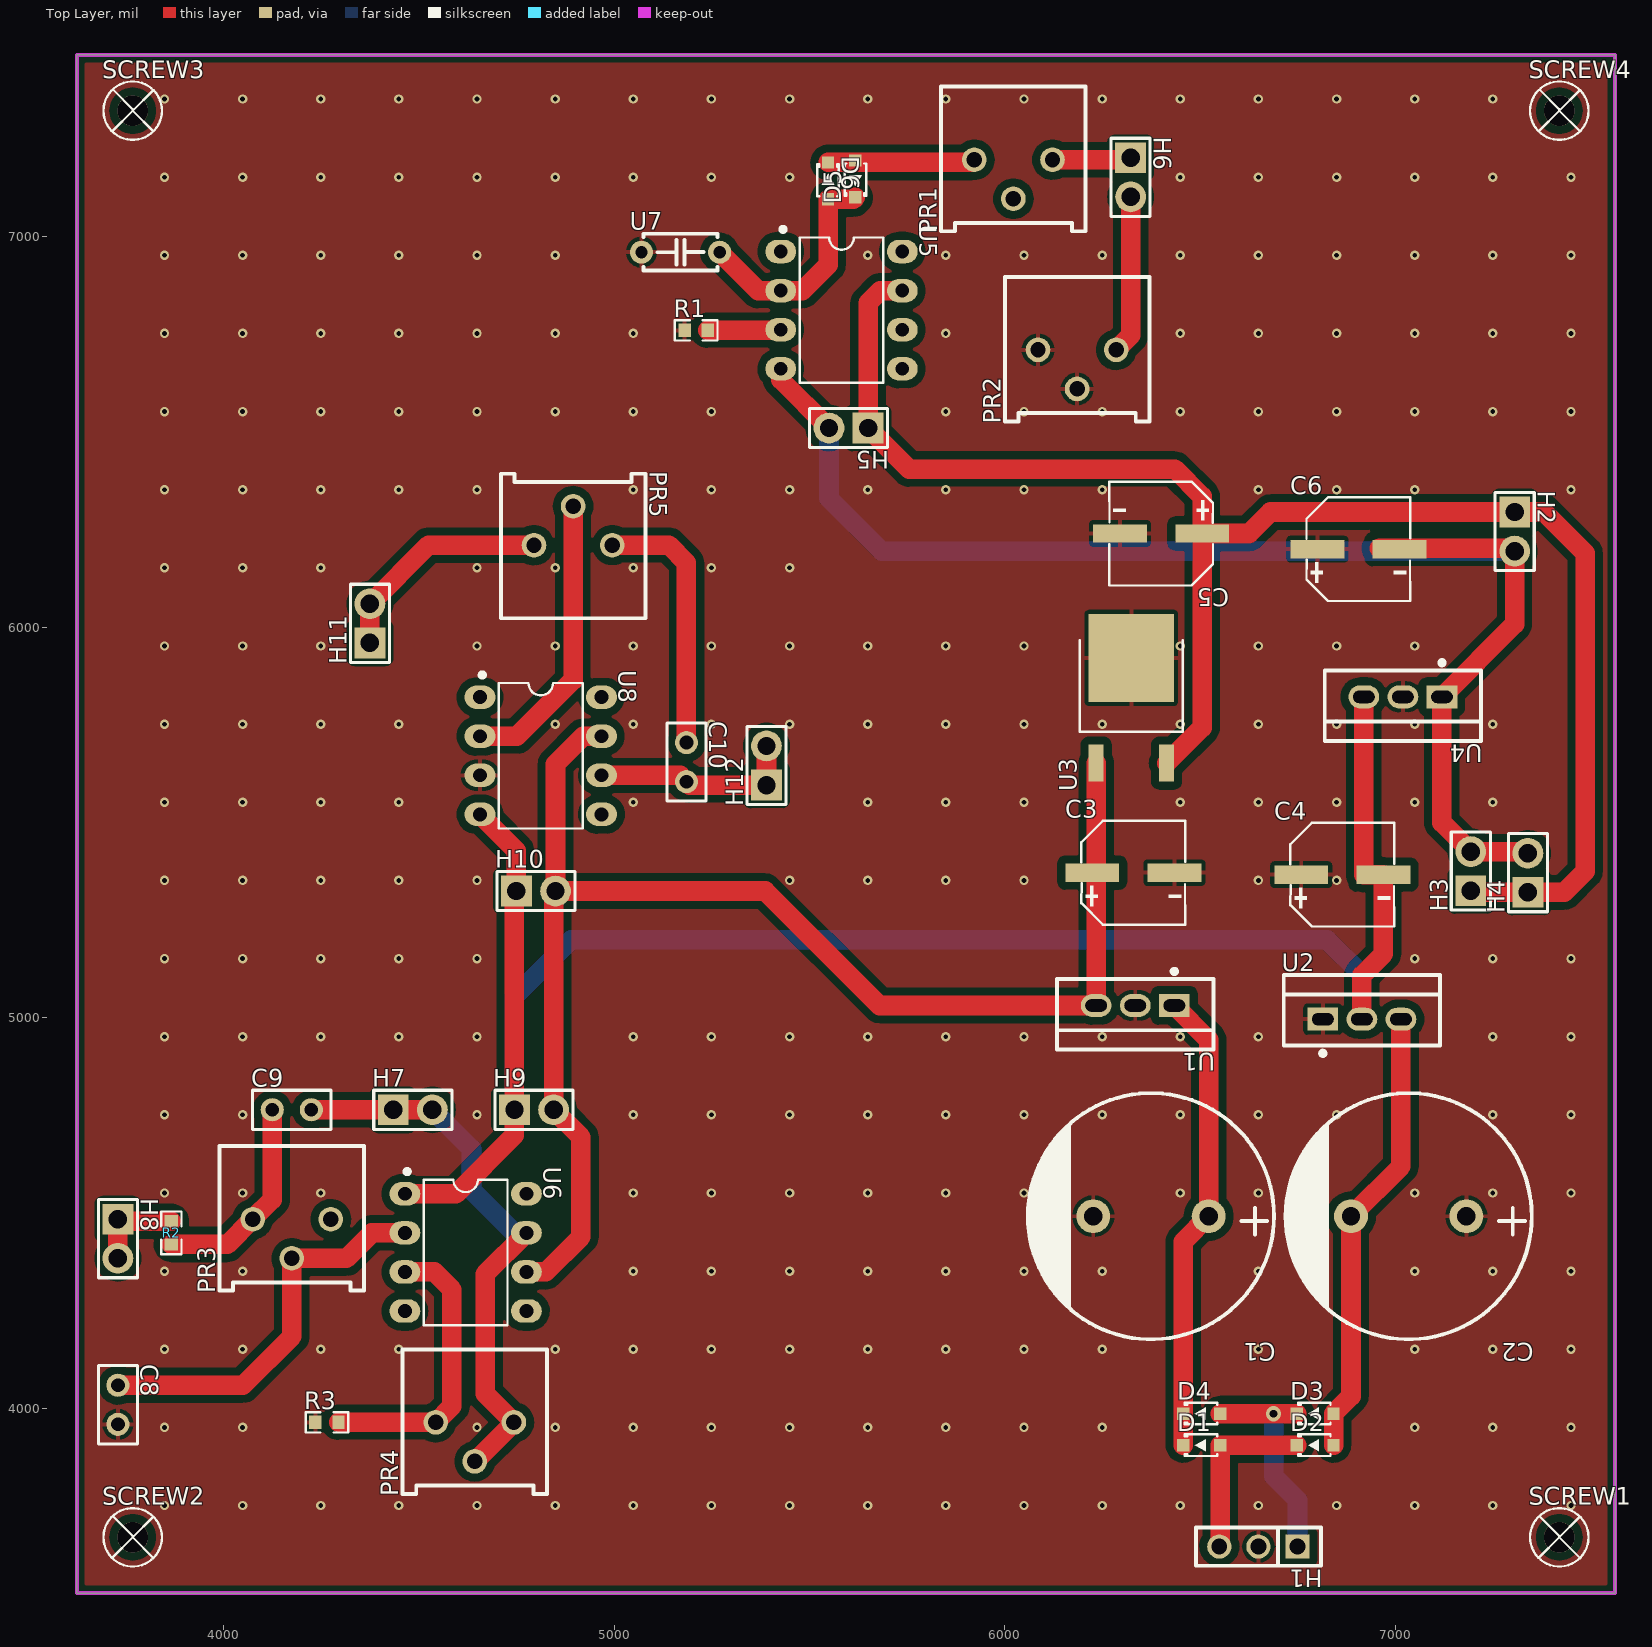
[diagram p0: Top Layer view]
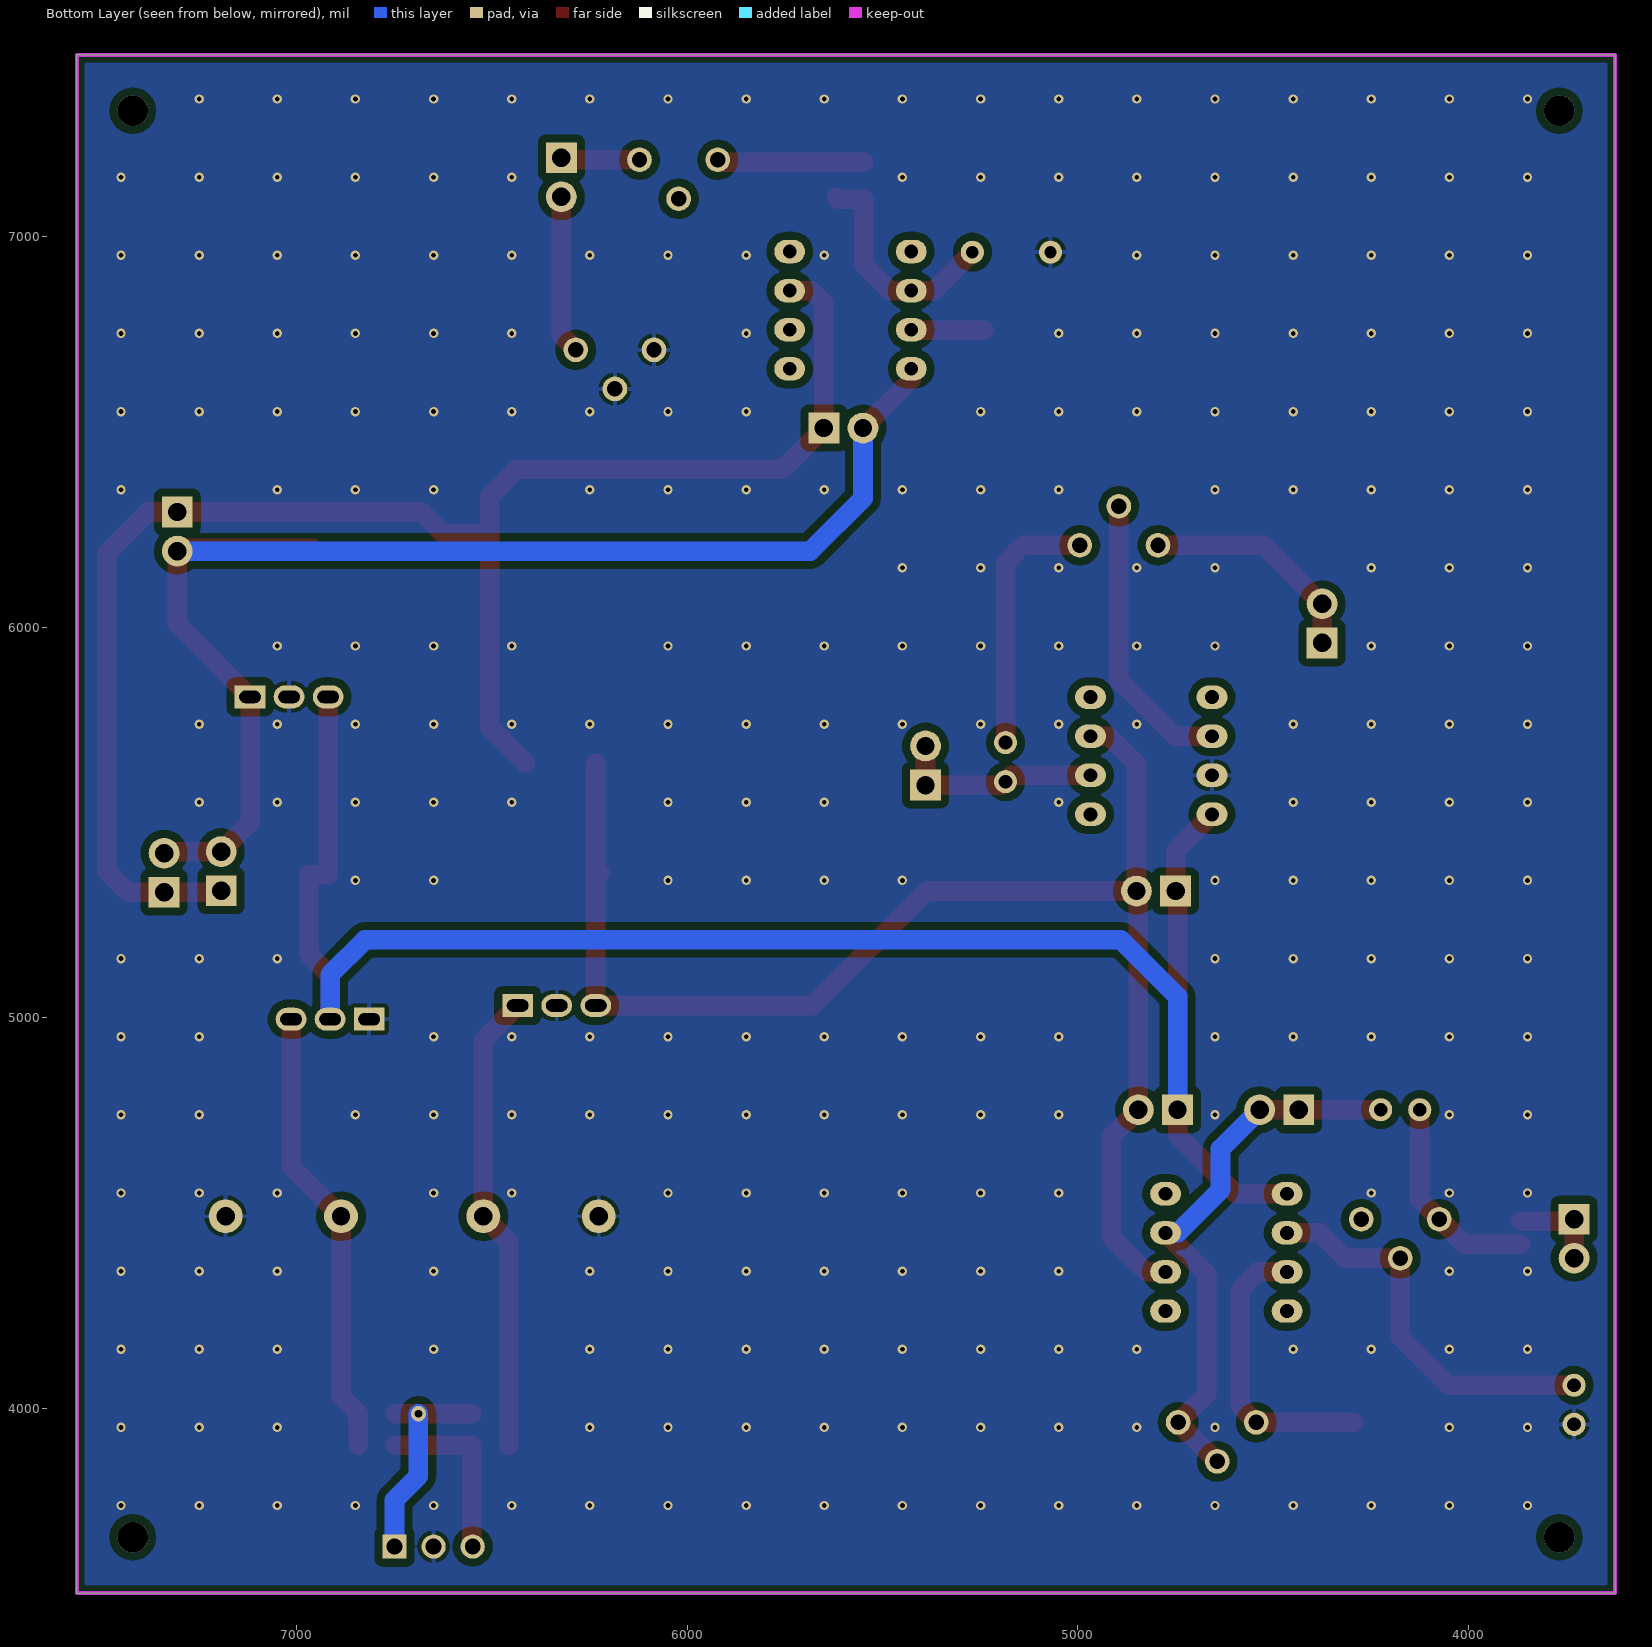
[diagram p1: Bottom Layer view, seen from below]
# Altium PCB MISC75076.pcbdoc
Units mil, origin at the board's own origin, x right, y up, seen from the top; angles counter-clockwise.
Board outline 3937.01 x 3937.01 mil, 2 copper layers (Top Layer, Bottom Layer), stack 62.206 mil thick; 47 components, 23 nets, 118 pads, 276 vias.

## Layer stack, top to bottom
Top Solder Mask Layer: solder mask 0.394, Dk 3.3
Top Layer: signal copper 1.379
Dielectric1: surface 59.449, FR4, Dk 4.5
Bottom Layer: signal copper 1.378
Bottom Solder Mask Layer: solder mask 0.394, Dk 3.3

## Board outline
3625,7465 3625,3527.99 7562.01,3527.99 7562.01,7465

## Design rules (kind name [scope] priority, off if disabled: settings)
BoardOutlineClearance copperThickness2oz_1 [All] p2 off: genericclearance=8 ignorepadtopadclearanceinfootprint=FALSE except(0: Arc-SplitContinuation Track-SplitContinuation SMDPad-SplitContinuation THPad-SplitContinuation Via-SplitContinuation Fill-SplitContinuation Region-SplitContinuation Poly-SplitContinuation Text-SplitContinuation Hole-SplitContinuation; 6: Arc-CutoutEdge Track-CutoutEdge SMDPad-CutoutEdge THPad-CutoutEdge Via-CutoutEdge Text-CutoutEdge; 6.9: Hole-OutlineEdge Hole-CutoutEdge; 11.8: Arc-OutlineEdge Track-OutlineEdge SMDPad-OutlineEdge THPad-OutlineEdge Via-OutlineEdge Fill-OutlineEdge Region-OutlineEdge Text-OutlineEdge Fill-CutoutEdge Region-CutoutEdge; 20: Poly-OutlineEdge Poly-CutoutEdge)
BoardOutlineClearance Copper_copperRegion_1 [All] p4 off: genericclearance=8 ignorepadtopadclearanceinfootprint=FALSE except(0: Arc-SplitContinuation Track-SplitContinuation SMDPad-SplitContinuation THPad-SplitContinuation Via-SplitContinuation Fill-SplitContinuation Region-SplitContinuation Poly-SplitContinuation Text-SplitContinuation Hole-SplitContinuation; 8: Arc-OutlineEdge Track-OutlineEdge SMDPad-OutlineEdge THPad-OutlineEdge Via-OutlineEdge Fill-OutlineEdge Region-OutlineEdge Text-OutlineEdge Hole-OutlineEdge Arc-CutoutEdge Track-CutoutEdge SMDPad-CutoutEdge THPad-CutoutEdge Via-CutoutEdge Fill-CutoutEdge Region-CutoutEdge Text-CutoutEdge Hole-CutoutEdge; 20: Poly-OutlineEdge Poly-CutoutEdge)
BoardOutlineClearance Plane_innerPlane_1 [All] p6 off: genericclearance=8 ignorepadtopadclearanceinfootprint=FALSE except(0: Arc-SplitContinuation Track-SplitContinuation SMDPad-SplitContinuation THPad-SplitContinuation Via-SplitContinuation Fill-SplitContinuation Region-SplitContinuation Poly-SplitContinuation Text-SplitContinuation Hole-SplitContinuation; 8: Arc-OutlineEdge Track-OutlineEdge SMDPad-OutlineEdge THPad-OutlineEdge Via-OutlineEdge Fill-OutlineEdge Region-OutlineEdge Text-OutlineEdge Hole-OutlineEdge Arc-CutoutEdge Track-CutoutEdge SMDPad-CutoutEdge THPad-CutoutEdge Via-CutoutEdge Fill-CutoutEdge Region-CutoutEdge Text-CutoutEdge Hole-CutoutEdge; 10: Poly-OutlineEdge Poly-CutoutEdge)
BoardOutlineClearance copperThickness1oz_1 [All] p8: genericclearance=8 ignorepadtopadclearanceinfootprint=FALSE except(0: Arc-SplitContinuation Track-SplitContinuation SMDPad-SplitContinuation THPad-SplitContinuation Via-SplitContinuation Fill-SplitContinuation Region-SplitContinuation Poly-SplitContinuation Text-SplitContinuation Hole-SplitContinuation; 8: Arc-OutlineEdge Track-OutlineEdge SMDPad-OutlineEdge THPad-OutlineEdge Via-OutlineEdge Fill-OutlineEdge Region-OutlineEdge Text-OutlineEdge Hole-OutlineEdge Arc-CutoutEdge Track-CutoutEdge SMDPad-CutoutEdge THPad-CutoutEdge Via-CutoutEdge Fill-CutoutEdge Region-CutoutEdge Text-CutoutEdge Hole-CutoutEdge; 20: Poly-OutlineEdge Poly-CutoutEdge)
Clearance copperThickness2oz [All] p1 off: gap=8 ignorepadtopadclearanceinfootprint=FALSE except(6: SMDPad-Track SMDPad-SMDPad THPad-Track SMDPad-THPad THPad-THPad Track-Via SMDPad-Via THPad-Via Via-Via Fill-SMDPad Region-SMDPad Fill-THPad Region-THPad Fill-Via Region-Via Fill-Fill Fill-Region Region-Region Arc-Track Arc-SMDPad Arc-THPad Arc-Via Fill-Arc Region-Arc Arc-Arc Text-Track SMDPad-Text Text-THPad Text-Via Fill-Text Region-Text Arc-Text Text-Text; 6.9: Hole-Track Hole-SMDPad Hole-THPad Hole-Via Fill-Hole Region-Hole Hole-Arc Hole-Text; 11.8: Fill-Track Region-Track; 20: Poly-Track Poly-SMDPad Poly-THPad Poly-Via Poly-Fill Poly-Region Poly-Poly Poly-Arc Poly-Text Poly-Hole)
Clearance Copper_copperRegion [All] p3 off: gap=8 ignorepadtopadclearanceinfootprint=FALSE except(20: Poly-Track Poly-SMDPad Poly-THPad Poly-Via Poly-Fill Poly-Region Poly-Poly Poly-Arc Poly-Text Poly-Hole)
Clearance Plane_innerPlane [All] p5 off: gap=8 ignorepadtopadclearanceinfootprint=FALSE except(10: Poly-Track Poly-SMDPad Poly-THPad Poly-Via Poly-Fill Poly-Region Poly-Poly Poly-Arc Poly-Text Poly-Hole)
Clearance copperThickness1oz [All] p7: gap=8 ignorepadtopadclearanceinfootprint=FALSE except(20: Poly-Track Poly-SMDPad Poly-THPad Poly-Via Poly-Fill Poly-Region Poly-Poly Poly-Arc Poly-Text Poly-Hole)
DiffPairsRouting differentialPair [All] p1: maxlimit=6 minlimit=6 mostfreqgap=6 toplayer_minwidth=5 toplayer_prefwidth=10 toplayer_maxwidth=100 toplayer_mingap=6 toplayer_prefgap=6 toplayer_maxgap=6 bottomlayer_minwidth=5 bottomlayer_prefwidth=10 bottomlayer_maxwidth=100 bottomlayer_mingap=6 bottomlayer_prefgap=6 bottomlayer_maxgap=6 maxuncoupledlength=10
HoleToHoleClearance otherClearance [All] p1: gap=11.8 allowstackedmicrovias=TRUE
Length netLength [All] p1: minlimit=0 maxlimit=0
MatchedLengths netLengthTolerance [All] p1: tolerance=1000
PasteMaskExpansion pasteMaskExpansion [All] p1: expansion=0
PlaneConnect innerPlane [All] p1: planeconnectstyle=Relief reliefexpansion=20 reliefentries=4 reliefconductorwidth=10 reliefairgap=10
PolygonConnect copperRegion [(InNet('GND'))] p1: connectstyle=Relief reliefconductorwidth=10 reliefentries=4 polygonreliefangle="90 Angle" airgapwidth=10 via.connectstyle=Relief via.reliefconductorwidth=10 via.reliefentries=4 via.polygonreliefangle="90 Angle" via.airgapwidth=10
RoutingVias viaSize [All] p1: holewidth=12 width=24 viastyle="Through Hole" minholewidth=11.8 minwidth=19.7 maxholewidth=248 maxwidth=393.7
SolderMaskExpansion solderMaskExpansion [IsVia] p1: expansion=-1000 istentingtop=TRUE
SolderMaskExpansion solderMaskExpansion [All] p2: expansion=2 istentingtop=FALSE
Width copperThickness2oz_2 [(InNet('-5V') OR InNet('-12V') OR InNet('+5V') OR InNet('+12V'))] p1: maxlimit=100 minlimit=8 preferedwidth=10
Width "VCC and GND" [All] p2 off: maxlimit=30 minlimit=10 preferedwidth=30
Width copperThickness1oz_2 [All] p3: maxlimit=50 minlimit=8 preferedwidth=50

## Components (designator, comment, footprint, x,y, rotation, side; value= is the part's Value field where it differs from the comment)
C1 "2200uF" CAP-TH_BD16.0-P7.50-D0.8-FD 6374.05,4492.61 r180 top
C2 "2200uF" CAP-TH_BD16.0-P7.50-D0.8-FD 7033.66,4492.61 r180 top
C3 "330uF" CAP-SMD_BD6.3-L6.6-W6.6-LS7.2-FD_3 6328.86,5371.91 r0 top
C4 "330uF" CAP-SMD_BD6.3-L6.6-W6.6-LS7.2-FD_3 6863.86,5366.91 r0 top
C5 "100uF" CAP-SMD_BD6.3-L6.6-W6.6-LS7.3-FD-H7.7 6400,6240 r180 top
C6 "100uF" CAP-SMD_BD6.3-L6.6-W6.6-LS7.3-FD-H7.7 6905,6200 r0 top
C8 "100nF" CAP-TH_L5.0-W2.5-P2.54-D0.7 3730,4010 r270 top
C9 "100nF" CAP-TH_L5.0-W2.5-P2.54-D0.7 4175,4765.15 r0 top
C10 "100nF" CAP-TH_L5.0-W2.5-P2.54-D0.7 5185.2,5654.8 r270 top
D1 "1N4007WS" SOD-323_L1.7-W1.3-LS2.5-RD 6504.05,3906.62 r0 top
D2 "1N4007WS" SOD-323_L1.7-W1.3-LS2.5-RD 6794.05,3906.62 r0 top
D3 "1N4007WS" SOD-323_L1.7-W1.3-LS2.5-RD 6794.05,3987.4 r0 top
D4 "1N4007WS" SOD-323_L1.7-W1.3-LS2.5-RD 6504.05,3987.4 r0 top
D5 "1N4007WS" SOD-323_L1.7-W1.3-LS2.5-RD 5617.5,7147.5 r90 top
D6 "1N4007WS" SOD-323_L1.7-W1.3-LS2.5-RD 5547.5,7142.5 r270 top
H1 "PM254V-11-03-H85" HDR-TH_3P-P2.54-V-F 6649.05,3647.17 r180 top
H2 "HX PH254-01-02-Z-L11.5 male header connector" HDR-TH_2P-P2.54-V-M 7305,6245 r270 top
H3 "HX PH254-01-02-Z-L11.5 male header connector" HDR-TH_2P-P2.54-V-M 7192.74,5375.94 r90 top
H4 "HX PH254-01-02-Z-L11.5 male header connector" HDR-TH_2P-P2.54-V-M 7338.86,5371.91 r90 top
H5 "HX PH254-01-02-Z-L11.5 male header connector" HDR-TH_2P-P2.54-V-M 5600,6510 r180 top
H6 "HX PH254-01-02-Z-L11.5 male header connector" HDR-TH_2P-P2.54-V-M 6322,7151.59 r270 top
H7 "HX PH254-01-02-Z-L11.5 male header connector" HDR-TH_2P-P2.54-V-M 4484.93,4765 r0 top
H8 "HX PH254-01-02-Z-L11.5 male header connector" HDR-TH_2P-P2.54-V-M 3730,4435 r270 top
H9 "HX PH254-01-02-Z-L11.5 male header connector" HDR-TH_2P-P2.54-V-M 4795,4765 r0 top
H10 "HX PH254-01-02-Z-L11.5 male header connector" HDR-TH_2P-P2.54-V-M 4800,5325 r0 top
H11 "HX PH254-01-02-Z-L11.5 male header connector" HDR-TH_2P-P2.54-V-M 4375,6010 r90 top
H12 "HX PH254-01-02-Z-L11.5 male header connector" HDR-TH_2P-P2.54-V-M 5389.98,5646.15 r90 top
PR1 "5K" R_3386P 6022,7196.59 r90 top
PR2 "5K" R_3386P 6185,6710 r90 top
PR3 "1K" R_3386P 4175,4485 r90 top
PR4 "1K" R_3386P 4643.49,3965 r90 top
PR5 "2K" R_3386P 4895,6210 r270 top
R1 "1kΩ" R0603 5210,6760 r0 top
R2 "1kΩ" R0603 3866.78,4450 r270 top
R3 "1kΩ" R0603 4265,3965 r0 top
SCREW1 "" M2螺丝 7419.15,3670.85 r0 top
SCREW2 "" M2螺丝 3767.85,3670.85 r0 top
SCREW3 "" M2螺丝 3767.85,7322.15 r0 top
SCREW4 "" M2螺丝 7419.15,7322.15 r0 top
U1 "LM7812CT/NOPB" TO-220-3_L10.2-W4.6-P2.54-L 6333.86,5031.91 r180 top
U2 "LM7912CT/NOPB" TO-220-3_L10.2-W4.6-P2.54-L 6913.86,4996.91 r0 top
U3 "LM7805-5V" TO-252-2_L6.6-W6.1-P4.58-LS9.9-TL 6323.86,5786.91 r90 top
U4 "LM7812CT/NOPB" TO-220-3_L10.2-W4.6-P2.54-L 7018.86,5821.91 r180 top
U5 "LF411CP" PDIP-8_L9.3-W6.4-P2.54-LS7.9-BL-1 5582,6811.59 r270 top
U6 "LF411CP" PDIP-8_L9.3-W6.4-P2.54-LS7.9-BL-1 4620,4400 r270 top
U7 "470nF" CAP-TH_L4.8-W2.4-P5.08-D0.6 5170,6960 r0 top
U8 "LF411CP" PDIP-8_L9.3-W6.4-P2.54-LS7.9-BL-1 4812.25,5671.15 r270 top

## Footprints (in the part's own frame and the unit in brackets; to place one, negate y for a bottom-side part, rotate by r counter-clockwise, add the part's x,y. Pads: shape width x height; smd on the part's side, far side on the other; paste and mask are expansions set on the pad)
CAP-SMD_BD6.3-L6.6-W6.6-LS7.2-FD_3 [mm]
  rect 3.5x1.2 smd: 1(-2.67,0) 2(2.67,0)
  silkscreen extent -3.38,-3.38 3.38,3.38
CAP-SMD_BD6.3-L6.6-W6.6-LS7.3-FD-H7.7 [mm]
  rect 3.5x1.2 smd: 1(-2.67,0) 2(2.67,0)
  silkscreen extent -3.38,-3.38 3.38,3.38
CAP-TH_BD16.0-P7.50-D0.8-FD [mm]
  round 2.2 hole 1.2: 1(-3.75,0) 2(3.75,0)
  silkscreen extent -8,-8 8,8
CAP-TH_L4.8-W2.4-P5.08-D0.6 [mm]
  round 1.5 hole 0.8: 1(-2.54,0) 2(2.54,0)
  silkscreen extent -2.4,-1.2 2.4,1.2
CAP-TH_L5.0-W2.5-P2.54-D0.7 [mm]
  round 1.5 hole 0.9 paste+0 mask+0.05: 1(-1.27,0) 2(1.27,0)
  silkscreen extent -2.54,-1.27 2.54,1.27
HDR-TH_2P-P2.54-V-M [mm]
  rect 2x2 hole 1.2: 1(-1.27,0)
  round 2 hole 1.2: 2(1.27,0)
  silkscreen extent -2.54,-1.27 2.54,1.27
HDR-TH_3P-P2.54-V-F [mil]
  rect 62x62 hole 40.16: 1(-100,0)
  round 62 hole 40.16: 2(0,0) 3(100,0)
  silkscreen extent -160,-49 160,49
M2螺丝 [mm]
  round 2 hole 2: 1(0,0)
  silkscreen extent -1.9,-1.9 1.9,1.9
PDIP-8_L9.3-W6.4-P2.54-LS7.9-BL-1 [mm]
  oval 1.524x2 hole 0.9: 1(-3.81,-3.95) 2(-1.27,-3.95) 3(1.27,-3.95) 4(3.81,-3.95) 5(3.81,3.95) 6(1.27,3.95) 7(-1.27,3.95) 8(-3.81,3.95)
  silkscreen extent -5.4,-3.95 4.73,2.72
R0603 [mil]
  rect 31.75x34.02 smd paste-3937.01 mask+2: 1(-29.66,0) 2(29.66,0)
  silkscreen extent -55,-26 55,26
R_3386P [mil]
  round 63 hole 39.4 paste+0 mask+2: 1(0,-100) 2(-100,0) 3(0,100)
  silkscreen extent -183,-185 187,185
SOD-323_L1.7-W1.3-LS2.5-RD [mm]
  rect 0.8x0.8 smd: 1(-1.2,0) 2(1.2,0)
  silkscreen extent -1.1,-0.7 1,0.7
TO-220-3_L10.2-W4.6-P2.54-L [mm]
  rect 2x1.5 hole 0.8 slot 1.4 at 0 deg: 1(-2.54,0)
  oval 2x1.5 hole 0.8 slot 1.4 at 0 deg: 2(0,0) 3(2.54,0)
  silkscreen extent -5.08,-2.37 5.08,2.86
TO-252-2_L6.6-W6.1-P4.58-LS9.9-TL [mil]
  rect 94.84x38.53 smd: 1(-134.8,90.15) 3(-134.78,-90.16)
  rect 224.84x218.44 smd: 2(134.8,0.01)
  silkscreen extent -54,-132 180,132

## Via types
v1: diameter 24, hole 12, Top Layer to Bottom Layer, 275 vias
v2: diameter 39.37, hole 19.7, Top Layer to Bottom Layer, 1 vias

## Nets (pads, with @x,y where several pads share a name; then routed paths per layer and width w, separated by ;. In a path a pad name is that pad's centre, name@x,y a point inside that pad or via, vN(x,y) a via of type N, cw(c..) or ccw(c..) an arc to the next point about the centre after c; other vN are vias at no path point)
$1N34: D1.2 D2.1 H1.3 | length 455.9
  Top Layer w50: H1.3 6551.29,3649.41 D1.2 D2.1
$1N35: D3.1 D4.2 H1.1 | length 561.2
  Top Layer w50: D4.2 v2(6687.74,3987.4) D3.1
  Bottom Layer w50: v2(6687.74,3987.4) 6687.74,3827.26 6749.05,3765.95 H1.1
$1N37: C1.1 D1.1 D4.1 U1.1 | length 1188.5
  Top Layer w50: U1.1 6521.69,4944.07 C1.1 6456.81,4427.73 D4.1 D1.1
$1N38: C2.2 D2.2 D3.2 U2.3 | length 1161.8
  Top Layer w50: D2.2 D3.2 6886.02,4032.13 C2.2 7013.86,4620.44 U2.3
$1N53: D5.1 D6.2 U5.2 U7.2 | length 585.4
  Top Layer w50: U7.2 5368.41,6861.59 U5.2 5481.59,6861.59 5547.5,6927.5 D6.2 5612.5,7095.26 D5.1
$1N54: R1.2 U5.3 | length 187.5
  Top Layer w50: R1.2 5424.9,6760 U5.3
$1N60: H6.2 PR2.1 | length 406.9
  Top Layer w50: PR2.1 6322,6747 H6.2
$1N61: D5.2 D6.1 PR1.3 | length 377.3
  Top Layer w50: D6.1 5915.15,7189.74 PR1.3
$1N67: H8.1 H8.2 R2.1 | length 239
  Top Layer w50: H8.2 H8.1 3735.34,4479.66 R2.1
$1N68: C9.1 PR3.3 R2.2 | length 535.9
  Top Layer w50: R2.2 4010.34,4420.34 PR3.3 4125,4535 C9.1
$1N70: PR4.3 R3.2 U6.3 | length 745.2
  Top Layer w50: R3.2 PR4.3 4585,4006.51 4585,4305 4540,4350 U6.3
$1N71: C8.1 PR3.2 U6.2 | length 1013.2
  Top Layer w50: C8.1 4050,4060 4175,4185 PR3.2 4315,4385 4380,4450 U6.2
$1N79: PR5.2 U8.2 | length 742.8
  Top Layer w50: U8.2 4751.15,5721.15 4895,5865 PR5.2
$1N80: H11.1 H11.2 PR5.1 | length 582.1
  Top Layer w50: H11.1 H11.2 4525,6210 PR5.1
$1N81: C10.1 PR5.3 | length 668.9
  Top Layer w50: PR5.3 5140,6210 5185.2,6164.8 C10.1
+5V: C5.1 H2.1 H3.1 H4.1 H5.1 U3.3 U5.7 | length 4245.8
  Top Layer w50: U5.7 5681.59,6861.59 5650,6830 H5.1 5755,6405 6435,6405 6505.12,6334.88 C5.1 ; U3.3 6505.12,5743.24 C5.1 ; H3.1 7196.77,5321.91 H4.1 7431.91,5321.91 7485,5375 7485,6190 7380,6295 H2.1 6680,6295 6625,6240 C5.1
+12V: C3.1 H9.2 H10.2 U1.3 U3.1 U6.6 U8.7 | length 3704.7
  Top Layer w50: U6.6 4825,4350 4915,4440 4915,4695 H9.2 4845,5320 H10.2 ; U8.7 4921.15,5721.15 4850,5650 H10.2 ; C3.1 C3.1@6233.7,5381.87 ; U3.1 C3.1@6233.7,5381.87 ; H10.2 5386.25,5325 5679.34,5031.92 U1.3 6233.7,5032.07 C3.1@6233.7,5381.87
-5V: C6.2 H2.2 H3.2 H4.2 H5.2 U4.1 U5.4 | length 3567.1
  Top Layer w50: U5.4 5426.49,6633.51 H5.2 ; C6.2@6958.98,6201.91 7298.09,6201.91 H2.2 7305,6008.05 U4.1 7118.85,5499.83 H3.2 7334.82,5425.94 H4.2
  Bottom Layer w50: H5.2 5550,6330 5685,6195 H2.2
-12V: C4.2 H9.1 H10.1 U2.2 U4.3 U6.1 U8.4 | length 4772.4
  Top Layer w50: U6.1 4595,4550 4745,4700 H9.1 4745,5320 H10.1 4750,5427.88 U8.4 ; U2.2 6913.86,5108.86 6968.97,5163.97 C4.2 6918.85,5366.91 U4.3
  Bottom Layer w50: H9.1 4745,5055 4890,5200 6825,5200 6913.86,5111.14 U2.2
GND: C1.2 C2.1 C3.2 C4.1 C5.2 C6.1 C8.2 H1.2 PR2.2 PR2.3 R1.1 R3.1 U1.2 U2.1 U3.2 U4.2 U7.1 U8.3
  other v1: 3849.1,3752.09 4049.1,3752.09 4249.1,3752.09 4449.1,3752.09 4649.1,3752.09 4849.1,3752.09 5049.1,3752.09 5249.1,3752.09 5449.1,3752.09 5649.1,3752.09 5849.1,3752.09 6049.1,3752.09 6249.1,3752.09 6449.1,3752.09 6649.1,3752.09 6849.1,3752.09 7049.1,3752.09 7249.1,3752.09 7449.1,3752.09 3849.1,3952.09 4049.1,3952.09 4649.1,3952.09 4849.1,3952.09 5049.1,3952.09 5249.1,3952.09 5449.1,3952.09 5649.1,3952.09 5849.1,3952.09 6049.1,3952.09 6249.1,3952.09 7049.1,3952.09 7249.1,3952.09 7449.1,3952.09 3849.1,4152.09 4049.1,4152.09 4249.1,4152.09 4449.1,4152.09 4849.1,4152.09 5049.1,4152.09 5249.1,4152.09 5449.1,4152.09 5649.1,4152.09 5849.1,4152.09 6049.1,4152.09 6249.1,4152.09 6649.1,4152.09 7049.1,4152.09 7249.1,4152.09 7449.1,4152.09 3849.1,4352.09 4049.1,4352.09 5049.1,4352.09 5249.1,4352.09 5449.1,4352.09 5649.1,4352.09 5849.1,4352.09 6049.1,4352.09 6249.1,4352.09 6649.1,4352.09 7049.1,4352.09 7249.1,4352.09 7449.1,4352.09 3849.1,4552.09 4049.1,4552.09 4249.1,4552.09 5049.1,4552.09 5249.1,4552.09 5449.1,4552.09 5649.1,4552.09 5849.1,4552.09 6049.1,4552.09 6449.1,4552.09 6649.1,4552.09 7049.1,4552.09 7249.1,4552.09 7449.1,4552.09 3849.1,4752.09 4049.1,4752.09 4649.1,4752.09 5049.1,4752.09 5249.1,4752.09 5449.1,4752.09 5649.1,4752.09 5849.1,4752.09 6049.1,4752.09 6249.1,4752.09 6449.1,4752.09 6649.1,4752.09 6849.1,4752.09 7249.1,4752.09 7449.1,4752.09 3849.1,4952.09 4049.1,4952.09 4249.1,4952.09 4449.1,4952.09 4649.1,4952.09 5049.1,4952.09 5249.1,4952.09 5449.1,4952.09 5649.1,4952.09 5849.1,4952.09 6049.1,4952.09 6249.1,4952.09 6449.1,4952.09 6649.1,4952.09 7249.1,4952.09 7449.1,4952.09 3849.1,5152.09 4049.1,5152.09 4249.1,5152.09 4449.1,5152.09 4649.1,5152.09 7049.1,5152.09 7249.1,5152.09 7449.1,5152.09 3849.1,5352.09 4049.1,5352.09 4249.1,5352.09 4449.1,5352.09 4649.1,5352.09 5449.1,5352.09 5649.1,5352.09 5849.1,5352.09 6049.1,5352.09 6649.1,5352.09 6849.1,5352.09 3849.1,5552.09 4049.1,5552.09 4249.1,5552.09 4449.1,5552.09 5049.1,5552.09 5649.1,5552.09 5849.1,5552.09 6049.1,5552.09 6449.1,5552.09 6649.1,5552.09 6849.1,5552.09 7049.1,5552.09 7249.1,5552.09 3849.1,5752.09 4049.1,5752.09 4249.1,5752.09 4449.1,5752.09 4849.1,5752.09 5049.1,5752.09 5249.1,5752.09 5449.1,5752.09 5649.1,5752.09 5849.1,5752.09 6049.1,5752.09 6249.1,5752.09 6449.1,5752.09 6649.1,5752.09 6849.1,5752.09 7049.1,5752.09 7249.1,5752.09 3849.1,5952.09 4049.1,5952.09 4249.1,5952.09 4649.1,5952.09 4849.1,5952.09 5049.1,5952.09 5249.1,5952.09 5449.1,5952.09 5649.1,5952.09 5849.1,5952.09 6049.1,5952.09 6449.1,5952.09 6649.1,5952.09 6849.1,5952.09 7049.1,5952.09 3849.1,6152.09 4049.1,6152.09 4249.1,6152.09 4649.1,6152.09 4849.1,6152.09 5049.1,6152.09 5249.1,6152.09 5449.1,6152.09 3849.1,6352.09 4049.1,6352.09 4249.1,6352.09 4449.1,6352.09 4649.1,6352.09 5049.1,6352.09 5249.1,6352.09 5449.1,6352.09 5649.1,6352.09 5849.1,6352.09 6049.1,6352.09 6249.1,6352.09 6649.1,6352.09 6849.1,6352.09 7049.1,6352.09 7449.1,6352.09 3849.1,6552.09 4049.1,6552.09 4249.1,6552.09 4449.1,6552.09 4649.1,6552.09 4849.1,6552.09 5049.1,6552.09 5249.1,6552.09 5849.1,6552.09 6049.1,6552.09 6249.1,6552.09 6449.1,6552.09 6649.1,6552.09 6849.1,6552.09 7049.1,6552.09 7249.1,6552.09 7449.1,6552.09 3849.1,6752.09 4049.1,6752.09 4249.1,6752.09 4449.1,6752.09 4649.1,6752.09 4849.1,6752.09 5049.1,6752.09 5849.1,6752.09 6449.1,6752.09 6649.1,6752.09 6849.1,6752.09 7049.1,6752.09 7249.1,6752.09 7449.1,6752.09 3849.1,6952.09 4049.1,6952.09 4249.1,6952.09 4449.1,6952.09 4649.1,6952.09 4849.1,6952.09 5649.1,6952.09 5849.1,6952.09 6049.1,6952.09 6249.1,6952.09 6449.1,6952.09 6649.1,6952.09 6849.1,6952.09 7049.1,6952.09 7249.1,6952.09 7449.1,6952.09 3849.1,7152.09 4049.1,7152.09 4249.1,7152.09 4449.1,7152.09 4649.1,7152.09 4849.1,7152.09 5049.1,7152.09 5249.1,7152.09 5449.1,7152.09 6449.1,7152.09 6649.1,7152.09 6849.1,7152.09 7049.1,7152.09 7249.1,7152.09 7449.1,7152.09 3849.1,7352.09 4049.1,7352.09 4249.1,7352.09 4449.1,7352.09 4649.1,7352.09 4849.1,7352.09 5049.1,7352.09 5249.1,7352.09 5449.1,7352.09 5649.1,7352.09 5849.1,7352.09 6049.1,7352.09 6249.1,7352.09 6449.1,7352.09 6649.1,7352.09 6849.1,7352.09 7049.1,7352.09 7249.1,7352.09
OUT1: H6.1 PR1.1 | length 202.1
  Top Layer w50: PR1.1 6317,7196.59 H6.1
OUT2: C10.2 H12.1 H12.2 U8.6 | length 532.6
  Top Layer w50: U8.6 5168.85,5621.15 C10.2 5193.85,5596.15 H12.1 H12.2
OUT3: C9.2 H7.1 H7.2 PR4.1 PR4.2 U6.7 | length 1443.1
  Top Layer w50: C9.2 4225.15,4765 H7.1 H7.2 ; PR4.2 PR4.1 4670,4038.49 4670,4344.49 U6.7
  Bottom Layer w50: H7.2 4635,4664.93 4635,4560 4745,4450 U6.7
pads on no net: PR1.2 PR3.1 SCREW1.1 SCREW2.1 SCREW3.1 SCREW4.1 U5.1 U5.5 U5.6 U5.8 U6.4 U6.5 U6.8 U8.1 U8.5 U8.8

## Polygon pours and split planes (outlines as drawn)
GND on Top Layer (solid, remove dead copper, pour order 0): 3000,7640 3000,3180 8080,3180 8080,7640
GND on Bottom Layer (solid, remove dead copper, pour order 2): 3095,7655 3095,3000 8160,3000 8160,7655

## Keep-outs
Board Outline Layer:
  the board outline again, w10